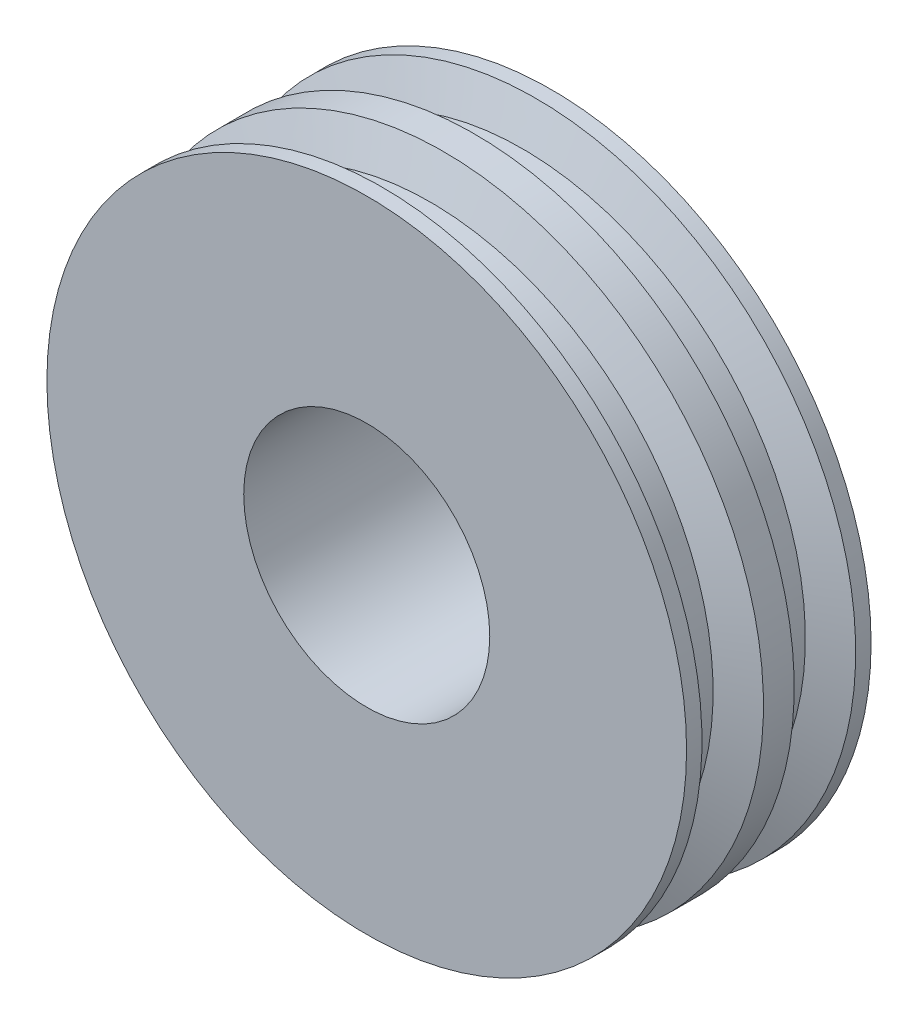
SolidWorks part; units mm, degrees
ref_plane "Front Plane" through (0, 0, 0) normal (0, 0, 1) x (1, 0, 0)
ref_plane "Top Plane" through (0, 0, 0) normal (0, 1, 0) x (1, 0, 0)
ref_plane "Right Plane" through (0, 0, 0) normal (1, 0, 0) x (0, 0, -1)
other "Configuration Table"
sketch "Sketch1" plane through (0, 0, 0) normal (0, 0, 1) x (1, 0, 0)
  circle A0 centre (0, 0) radius 52
  circle A1 centre (0, 0) radius 20
  dimension "D1" = 104
  dimension "D2" = 40
extrude "Boss-Extrude1" add sketch "Sketch1" along normal blind 30
sketch "Sketch2" plane through (0, 0, 0) normal (1, 0, 0) x (0, 0, -1)
  line L0 (-15, 52) -> (-15, -53.3396) construction
  line L1 (-25.3162, 46) -> (-19.6838, 46)
  line L6 (0, 0) -> (-55.6942, 0) construction
  line L10 (0, 52) -> (-30, 52) construction
  line L11 (-22.5, 57.3358) -> (-22.5, 27.6734) construction
  line L12 (-30, 52) -> (-30, -52) construction
  line L13 (-17.5, 52) -> (-27.5, 52)
  line L14 (-27.5, 52) -> (-25.3162, 46)
  line L15 (-17.5, 52) -> (-19.6838, 46)
  line L16 (-7.5, 57.3358) -> (-7.5, 27.6734) construction
  line L17 (-12.5, 52) -> (-10.3162, 46)
  line L18 (-2.5, 52) -> (-4.6838, 46)
  line L19 (-12.5, 52) -> (-2.5, 52)
  line L20 (-4.6838, 46) -> (-10.3162, 46)
  point P17 (-22.5, 46)
  point P18 (-22.5, 52)
  point P23 (-7.5, 52)
  point P24 (-7.5, 46)
  dimension "D1" = 7.5
  dimension "D2" = 10
  dimension "D3" = 6
  dimension "D4" = 40
revolve "Cut-Revolve1" cut sketch "Sketch2" angle 360 about L6
